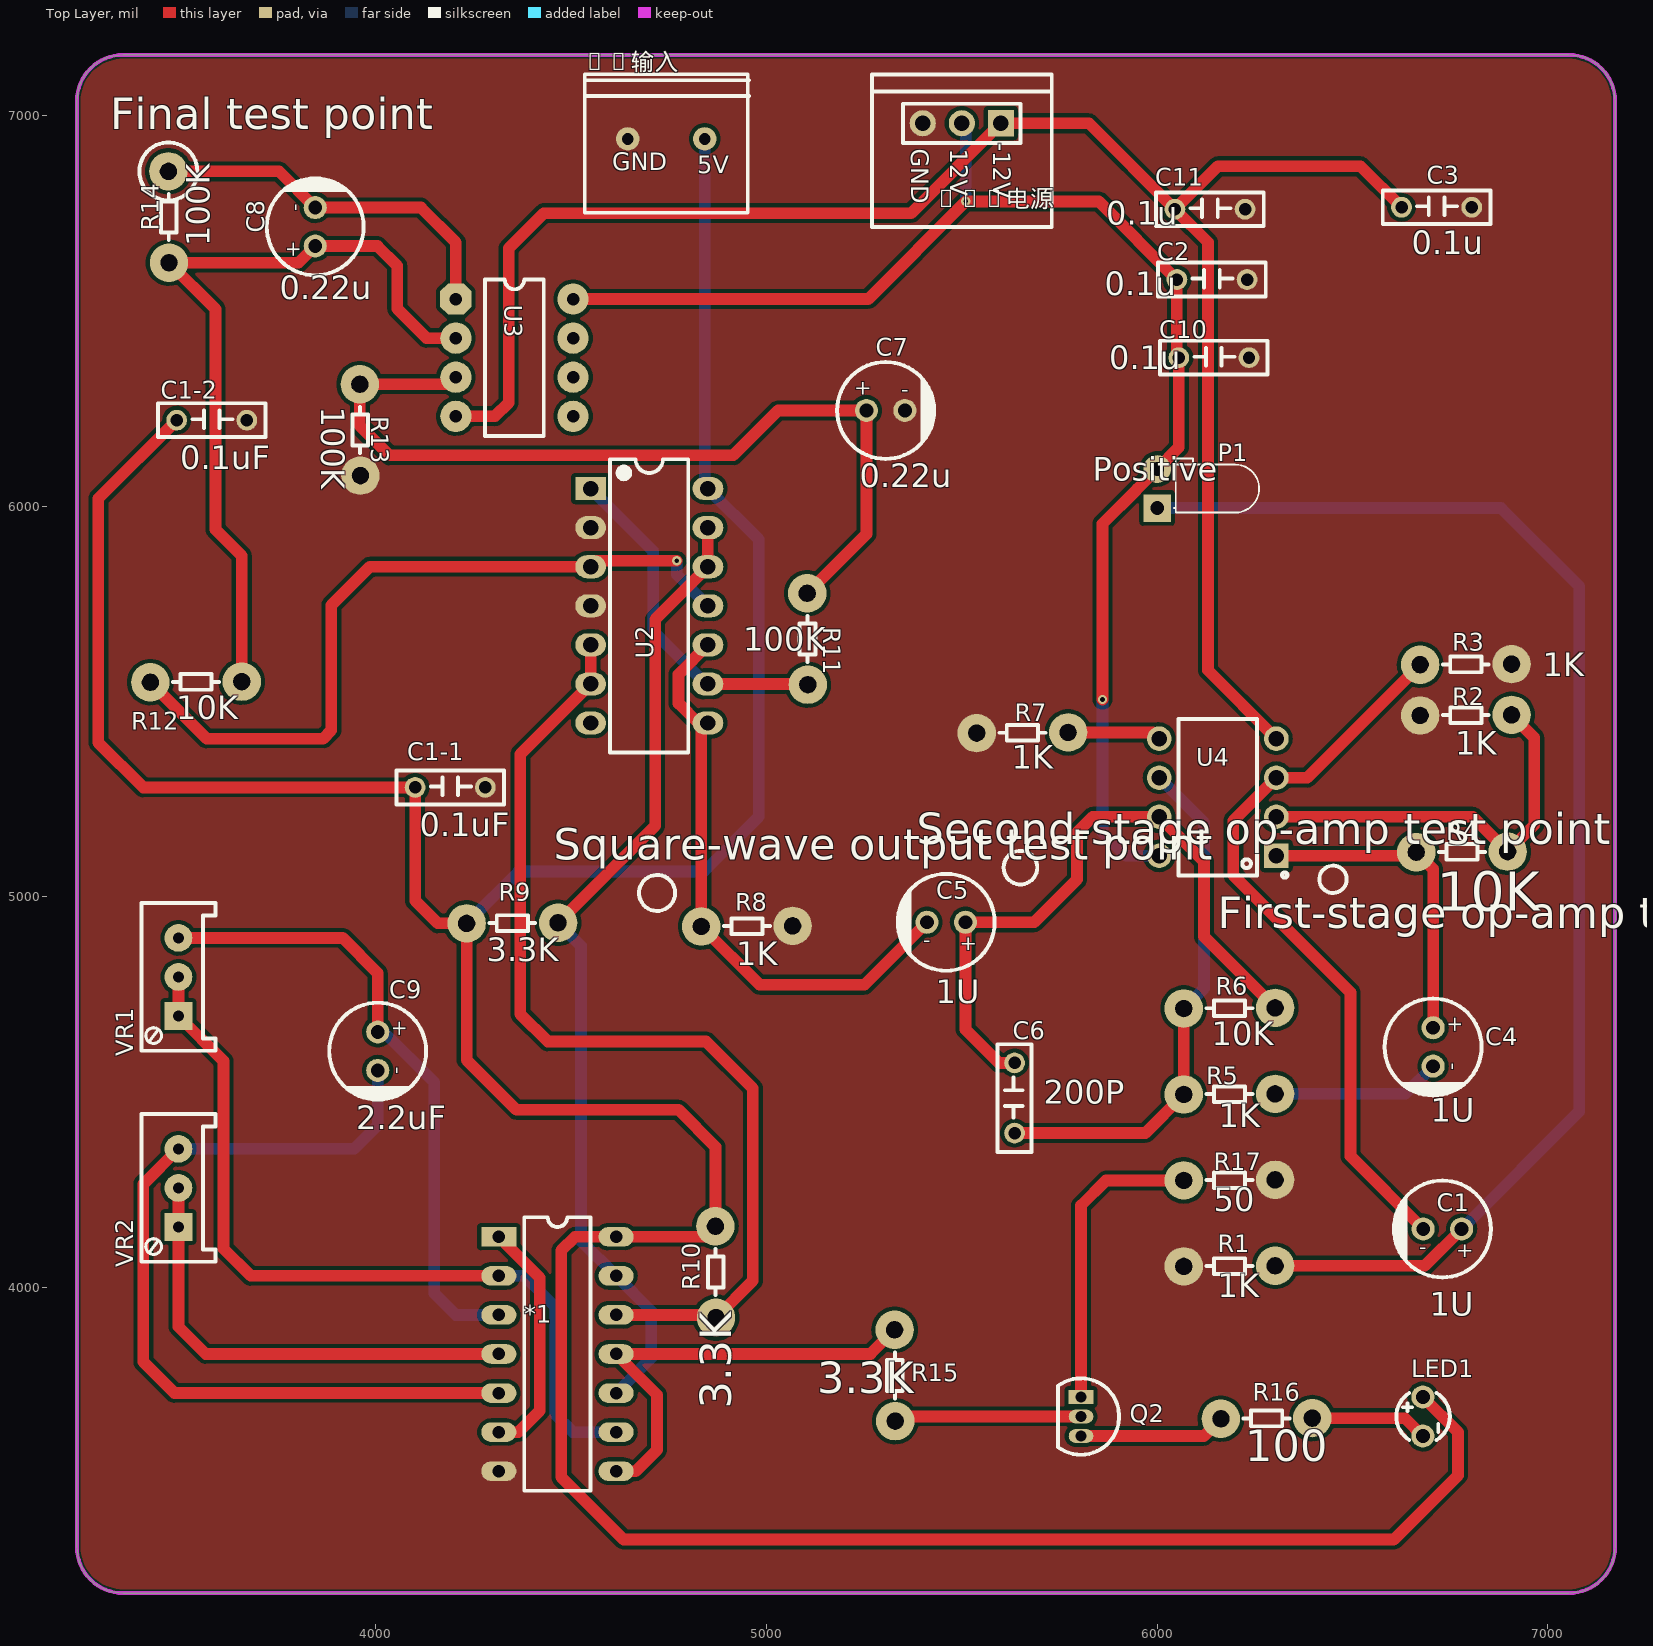
[diagram p0: Top Layer view]
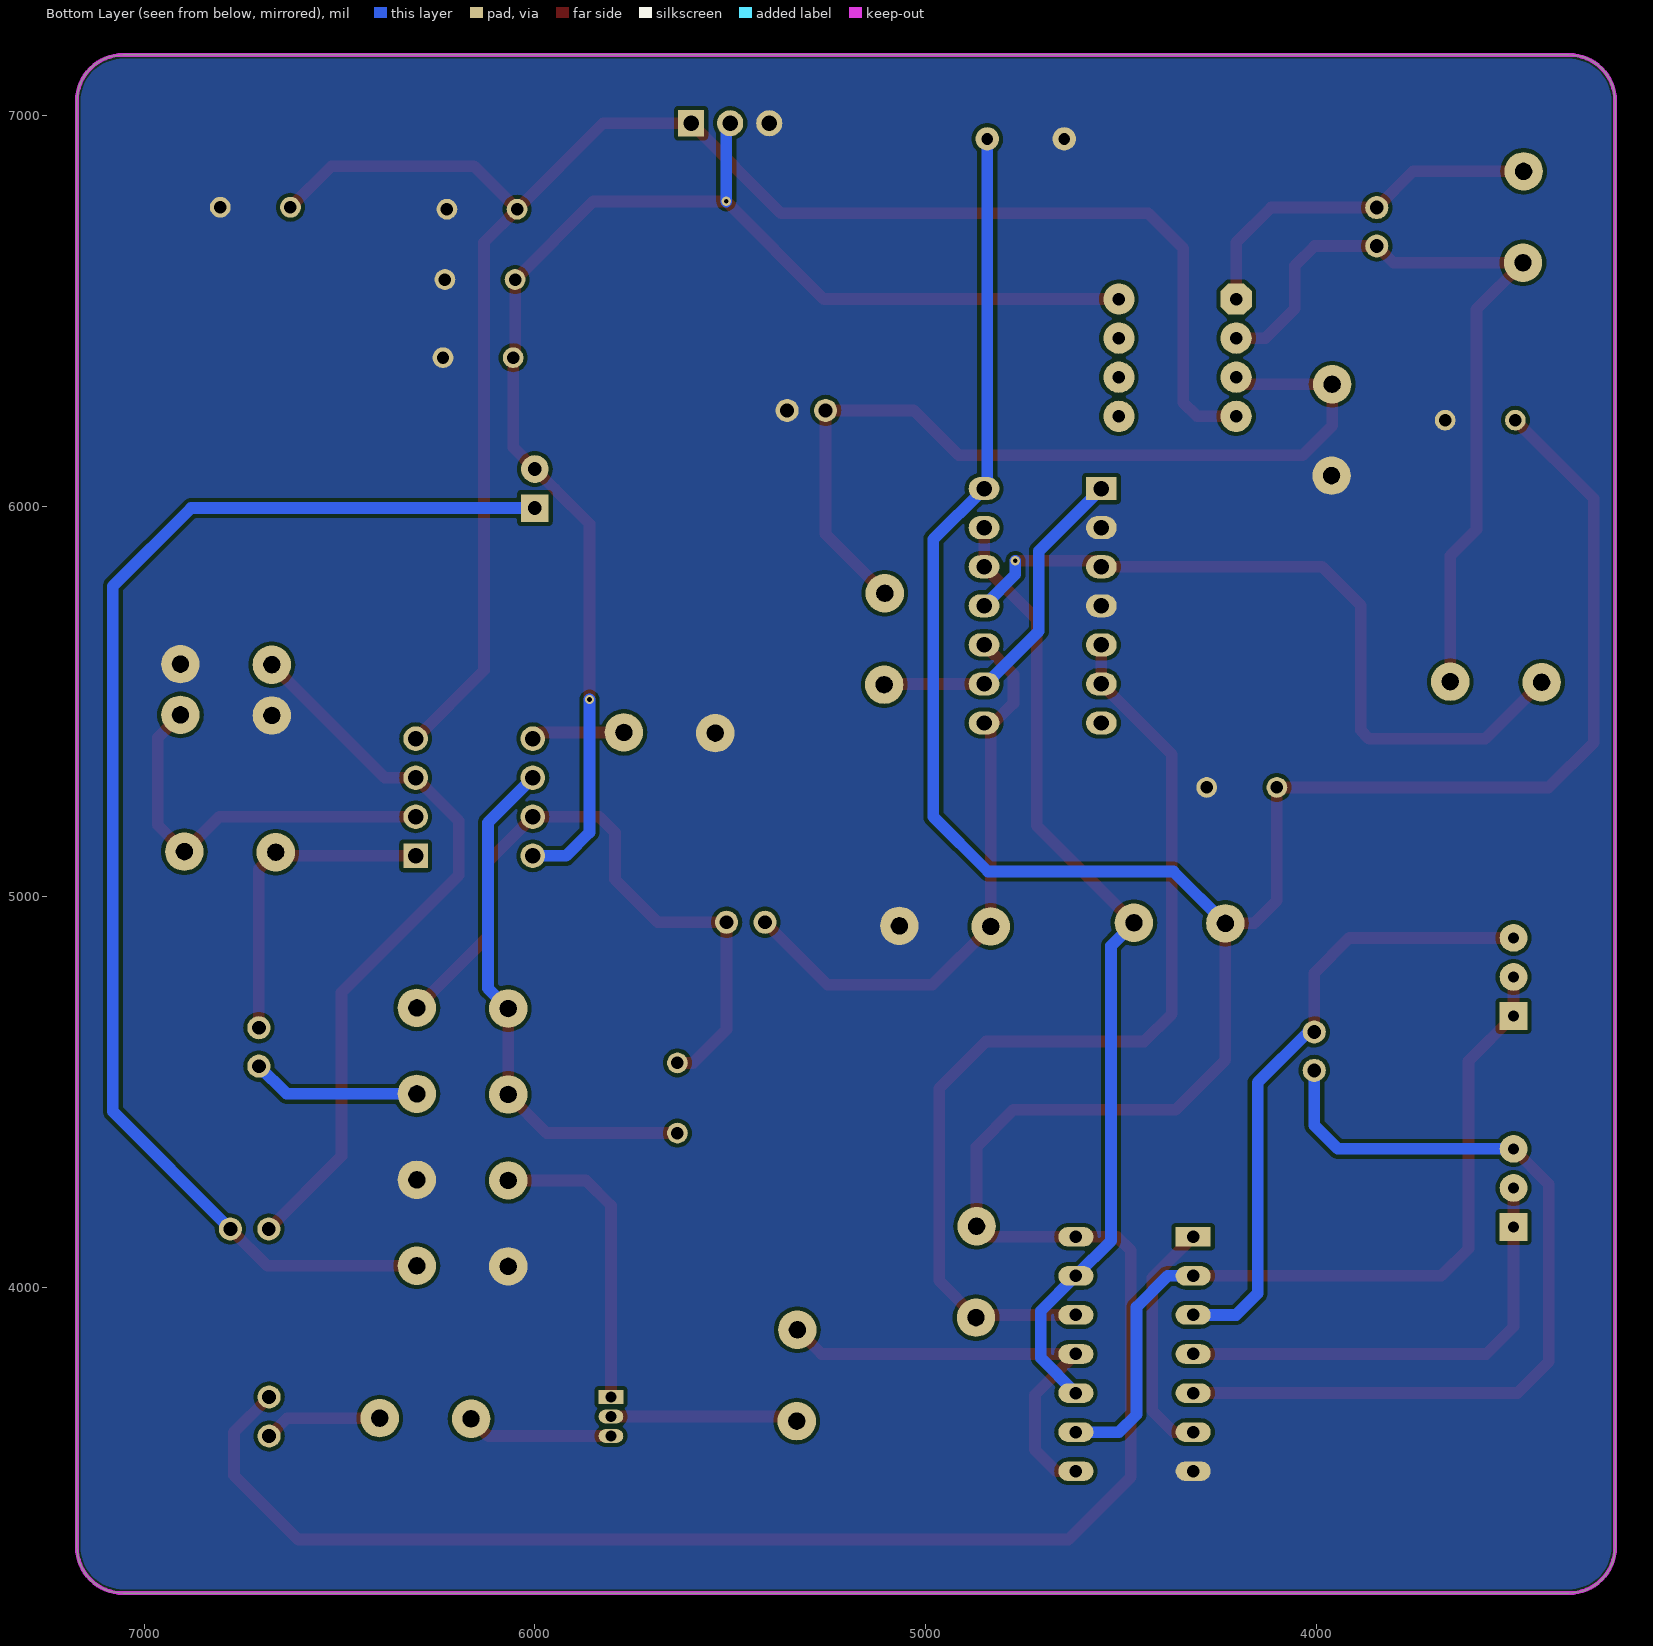
[diagram p1: Bottom Layer view, seen from below]
# Altium PCB MISC75396.pcbdoc
Units mil, origin at the board's own origin, x right, y up, seen from the top; angles counter-clockwise.
Board outline 3937.01 x 3937.01 mil, 2 copper layers (Top Layer, Bottom Layer), stack 62.206 mil thick; 41 components, 30 nets, 122 pads, 3 vias.

## Layer stack, top to bottom
Top Solder Mask Layer: solder mask 0.394, Dk 3.3
Top Layer: signal copper 1.379
Dielectric1: surface 59.449, FR4, Dk 4.5
Bottom Layer: signal copper 1.378
Bottom Solder Mask Layer: solder mask 0.394, Dk 3.3

## Board outline
3353.11,7155 ccw(c3353.11,7036.89) 3235,7036.89 3235,3336.1 ccw(c3353.11,3336.1) 3353.11,3217.99 7053.9,3217.99 ccw(c7053.9,3336.1) 7172.01,3336.1 7172.01,7036.89 ccw(c7053.9,7036.89) 7053.9,7155

## Design rules (kind name [scope] priority, off if disabled: settings)
BoardOutlineClearance copperThickness2oz_1 [All] p2 off: genericclearance=7.99 ignorepadtopadclearanceinfootprint=FALSE except(0: Arc-SplitContinuation Track-SplitContinuation SMDPad-SplitContinuation THPad-SplitContinuation Via-SplitContinuation Fill-SplitContinuation Region-SplitContinuation Poly-SplitContinuation Text-SplitContinuation Hole-SplitContinuation; 5.98: Arc-CutoutEdge Track-CutoutEdge SMDPad-CutoutEdge THPad-CutoutEdge Via-CutoutEdge Text-CutoutEdge; 6.89: Hole-OutlineEdge Hole-CutoutEdge; 10: Poly-OutlineEdge Poly-CutoutEdge; 11.81: Arc-OutlineEdge Track-OutlineEdge SMDPad-OutlineEdge THPad-OutlineEdge Via-OutlineEdge Fill-OutlineEdge Region-OutlineEdge Text-OutlineEdge Fill-CutoutEdge Region-CutoutEdge)
BoardOutlineClearance Plane_innerPlane_1 [All] p4 off: genericclearance=4.02 ignorepadtopadclearanceinfootprint=FALSE except(0: Arc-SplitContinuation Track-SplitContinuation SMDPad-SplitContinuation THPad-SplitContinuation Via-SplitContinuation Fill-SplitContinuation Region-SplitContinuation Poly-SplitContinuation Text-SplitContinuation Hole-SplitContinuation; 5.98: Arc-CutoutEdge Track-CutoutEdge SMDPad-CutoutEdge THPad-CutoutEdge Via-CutoutEdge Text-CutoutEdge; 6.89: Hole-OutlineEdge Hole-CutoutEdge; 10: Poly-OutlineEdge Poly-CutoutEdge; 11.81: Arc-OutlineEdge Track-OutlineEdge SMDPad-OutlineEdge THPad-OutlineEdge Via-OutlineEdge Fill-OutlineEdge Region-OutlineEdge Text-OutlineEdge Fill-CutoutEdge Region-CutoutEdge)
BoardOutlineClearance Copper_copperRegion_1 [All] p6 off: genericclearance=4.02 ignorepadtopadclearanceinfootprint=FALSE except(0: Arc-SplitContinuation Track-SplitContinuation SMDPad-SplitContinuation THPad-SplitContinuation Via-SplitContinuation Fill-SplitContinuation Region-SplitContinuation Poly-SplitContinuation Text-SplitContinuation Hole-SplitContinuation; 5.98: Arc-CutoutEdge Track-CutoutEdge SMDPad-CutoutEdge THPad-CutoutEdge Via-CutoutEdge Text-CutoutEdge; 6.89: Hole-OutlineEdge Hole-CutoutEdge; 10: Poly-OutlineEdge Poly-CutoutEdge; 11.81: Arc-OutlineEdge Track-OutlineEdge SMDPad-OutlineEdge THPad-OutlineEdge Via-OutlineEdge Fill-OutlineEdge Region-OutlineEdge Text-OutlineEdge Fill-CutoutEdge Region-CutoutEdge)
BoardOutlineClearance copperThickness1oz_1 [All] p8: genericclearance=4.02 ignorepadtopadclearanceinfootprint=FALSE except(0: Arc-SplitContinuation Track-SplitContinuation SMDPad-SplitContinuation THPad-SplitContinuation Via-SplitContinuation Fill-SplitContinuation Region-SplitContinuation Poly-SplitContinuation Text-SplitContinuation Hole-SplitContinuation; 5.98: Arc-CutoutEdge Track-CutoutEdge SMDPad-CutoutEdge THPad-CutoutEdge Via-CutoutEdge Text-CutoutEdge; 6.89: Hole-OutlineEdge Hole-CutoutEdge; 10: Poly-OutlineEdge Poly-CutoutEdge; 11.81: Arc-OutlineEdge Track-OutlineEdge SMDPad-OutlineEdge THPad-OutlineEdge Via-OutlineEdge Fill-OutlineEdge Region-OutlineEdge Text-OutlineEdge Fill-CutoutEdge Region-CutoutEdge)
Clearance copperThickness2oz [All] p1 off: gap=7.99 ignorepadtopadclearanceinfootprint=FALSE except(5.98: SMDPad-Track SMDPad-SMDPad THPad-Track SMDPad-THPad THPad-THPad Track-Via SMDPad-Via THPad-Via Via-Via Fill-SMDPad Region-SMDPad Fill-THPad Region-THPad Fill-Via Region-Via Fill-Fill Fill-Region Region-Region Arc-Track Arc-SMDPad Arc-THPad Arc-Via Fill-Arc Region-Arc Arc-Arc Text-Track SMDPad-Text Text-THPad Text-Via Fill-Text Region-Text Arc-Text Text-Text; 6.89: Hole-Track Hole-SMDPad Hole-THPad Hole-Via Fill-Hole Region-Hole Hole-Arc Hole-Text; 10: Poly-Track Poly-SMDPad Poly-THPad Poly-Via Poly-Fill Poly-Region Poly-Poly Poly-Arc Poly-Text Poly-Hole; 11.81: Fill-Track Region-Track)
Clearance Plane_innerPlane [All] p3 off: gap=4.02 ignorepadtopadclearanceinfootprint=FALSE except(5.98: SMDPad-Track SMDPad-SMDPad THPad-Track SMDPad-THPad THPad-THPad Track-Via SMDPad-Via THPad-Via Via-Via Fill-SMDPad Region-SMDPad Fill-THPad Region-THPad Fill-Via Region-Via Fill-Fill Fill-Region Region-Region Arc-Track Arc-SMDPad Arc-THPad Arc-Via Fill-Arc Region-Arc Arc-Arc Text-Track SMDPad-Text Text-THPad Text-Via Fill-Text Region-Text Arc-Text Text-Text; 6.89: Hole-Track Hole-SMDPad Hole-THPad Hole-Via Fill-Hole Region-Hole Hole-Arc Hole-Text; 10: Poly-Track Poly-SMDPad Poly-THPad Poly-Via Poly-Fill Poly-Region Poly-Poly Poly-Arc Poly-Text Poly-Hole; 11.81: Fill-Track Region-Track)
Clearance Copper_copperRegion [All] p5 off: gap=4.02 ignorepadtopadclearanceinfootprint=FALSE except(5.98: SMDPad-Track SMDPad-SMDPad THPad-Track SMDPad-THPad THPad-THPad Track-Via SMDPad-Via THPad-Via Via-Via Fill-SMDPad Region-SMDPad Fill-THPad Region-THPad Fill-Via Region-Via Fill-Fill Fill-Region Region-Region Arc-Track Arc-SMDPad Arc-THPad Arc-Via Fill-Arc Region-Arc Arc-Arc Text-Track SMDPad-Text Text-THPad Text-Via Fill-Text Region-Text Arc-Text Text-Text; 6.89: Hole-Track Hole-SMDPad Hole-THPad Hole-Via Fill-Hole Region-Hole Hole-Arc Hole-Text; 10: Poly-Track Poly-SMDPad Poly-THPad Poly-Via Poly-Fill Poly-Region Poly-Poly Poly-Arc Poly-Text Poly-Hole; 11.81: Fill-Track Region-Track)
Clearance copperThickness1oz [All] p7: gap=4.02 ignorepadtopadclearanceinfootprint=FALSE except(5.98: SMDPad-Track SMDPad-SMDPad THPad-Track SMDPad-THPad THPad-THPad Track-Via SMDPad-Via THPad-Via Via-Via Fill-SMDPad Region-SMDPad Fill-THPad Region-THPad Fill-Via Region-Via Fill-Fill Fill-Region Region-Region Arc-Track Arc-SMDPad Arc-THPad Arc-Via Fill-Arc Region-Arc Arc-Arc Text-Track SMDPad-Text Text-THPad Text-Via Fill-Text Region-Text Arc-Text Text-Text; 6.89: Hole-Track Hole-SMDPad Hole-THPad Hole-Via Fill-Hole Region-Hole Hole-Arc Hole-Text; 10: Poly-Track Poly-SMDPad Poly-THPad Poly-Via Poly-Fill Poly-Region Poly-Poly Poly-Arc Poly-Text Poly-Hole; 11.81: Fill-Track Region-Track)
DiffPairsRouting differentialPair [All] p1: maxlimit=6 minlimit=6 mostfreqgap=6 toplayer_minwidth=5 toplayer_prefwidth=10 toplayer_maxwidth=100 toplayer_mingap=6 toplayer_prefgap=6 toplayer_maxgap=6 bottomlayer_minwidth=5 bottomlayer_prefwidth=10 bottomlayer_maxwidth=100 bottomlayer_mingap=6 bottomlayer_prefgap=6 bottomlayer_maxgap=6 maxuncoupledlength=10
HoleToHoleClearance otherClearance [All] p1: gap=11.81 allowstackedmicrovias=TRUE
Length netLength [All] p1: minlimit=0 maxlimit=0
PasteMaskExpansion pasteMaskExpansion [All] p1: expansion=0
PlaneConnect innerPlane [All] p1: planeconnectstyle=Relief reliefexpansion=20 reliefentries=4 reliefconductorwidth=10 reliefairgap=10
PolygonConnect copperRegion [All] p1: connectstyle=Direct reliefconductorwidth=10 reliefentries=4 polygonreliefangle="90 Angle" airgapwidth=10 via.connectstyle=Relief via.reliefconductorwidth=10 via.reliefentries=4 via.polygonreliefangle="90 Angle" via.airgapwidth=10
RoutingVias viaSize [All] p1: holewidth=12.01 width=24.02 viastyle="Through Hole" minholewidth=11.81 minwidth=19.68 maxholewidth=248.03 maxwidth=393.7
SolderMaskExpansion solderMaskExpansion [IsVia] p1: expansion=-1000 istentingtop=TRUE
SolderMaskExpansion solderMaskExpansion [All] p2: expansion=2.01 istentingtop=FALSE
Width copperThickness2oz_2 [All] p1 off: maxlimit=100 minlimit=8 preferedwidth=10
Width copperThickness1oz_2 [All] p2: maxlimit=100 minlimit=5 preferedwidth=10

## Components (designator, comment, footprint, x,y, rotation, side; value= is the part's Value field where it differs from the comment)
5V输入 "5V output" 2INT 4645,6940 r0 top
12V电源 "3PIN" 3PIN 5500,6980 r0 top
*1 "74HC04" DIP14 4315.01,4129.99 r0 top
C1 "220uF" CAP-TH_BD6.3-P2.50-D0.5-FD 6730,4150 r180 top
C1-1 "" 电容直插 4190.33,5280.14 r180 top
C1-2 "" 电容直插 3580,6220 r180 top
C2 "" 电容直插 6140,6580 r180 top
C3 "" 电容直插 6715,6765 r180 top
C4 "220uF" CAP-TH_BD6.3-P2.50-D0.5-FD 6706.2,4615.85 r270 top
C5 "220uF" CAP-TH_BD6.3-P2.50-D0.5-FD 5460,4935 r180 top
C6 "" 电容直插 5635,4485 r270 top
C7 "220uF" CAP-TH_BD6.3-P2.50-D0.5-FD 5305,6245 r0 top
C8 "220uF" CAP-TH_BD6.3-P2.50-D0.5-FD 3845,6715 r90 top
C9 "220uF" CAP-TH_BD6.3-P2.50-D0.5-FD 4005,4605 r270 top
C10 "" 电容直插 6145,6380 r180 top
C11 "" 电容直插 6135,6760 r180 top
LED1 "3A4GUD" LED-TH_BD3.5-P2.54-RD-GREEN 6680,3670 r90 top
P1 "" LED_D3.0mm_Horizontal_O1.27mm_Z2.0mm 6000,6045 r90 top
Q2 "S9018" TO-92-3_L4.9-W3.7-P1.27-L 5805,3670 r270 top
R1 "" D45-V(直插) 6185,4055 r180 top
R2 "" D45-V(直插) 6790,5595 r0 top
R3 "" D45-V(直插) 6790,5465 r180 top
R4 "" D45-V(直插) 6780,5115 r0 top
R5 "" D45-V(直插) 6185,4495 r0 top
R6 "" D45-V(直插) 6185,4715 r0 top
R7 "" D45-V(直插) 5655,5420 r0 top
R8 "" D45-V(直插) 4950,4925 r0 top
R9 "" D45-V(直插) 4349.56,4932.93 r180 top
R10 "" D45-V(直插) 4870.01,4039.99 r90 top
R11 "" D45-V(直插) 5105,5660 r90 top
R12 "" D45-V(直插) 3540,5550 r0 top
R13 "" D45-V(直插) 3960,6195 r270 top
R14 "" D45-V(直插) 3470,6740 r90 top
R15 "" D45-V(直插) 5328.75,3775 r270 top
R16 "" D45-V(直插) 6280,3665 r0 top
R17 "" D45-V(直插) 6185,4275 r180 top
U2 "CD4066DN" PDIP-14_L19.3-W6.5-P2.54-LS7.6-BL 4700,5745 r270 top
U3 "LF353" DIP-8 4205,6530 r0 top
U4 "" DIP-8_L9.9-W6.4-P2.54-LS7.6-BL 6155,5255 r90 top
VR1 "101" 3296W 3495,4795 r90 top
VR2 "101" 3296W 3495,4255 r90 top

## Footprints (in the part's own frame and the unit in brackets; to place one, negate y for a bottom-side part, rotate by r counter-clockwise, add the part's x,y. Pads: shape width x height; smd on the part's side, far side on the other; paste and mask are expansions set on the pad)
2INT [mil]
  round 60 hole 30: 1(196.85,0) 2(0,0)
  silkscreen extent -110,-189 310,165
3PIN [mm]
  rect 1.7x1.7 hole 1: 1(2.54,0)
  round 1.7 hole 1: 2(0,0) 3(-2.54,0)
  silkscreen extent -3.84,-1.27 3.81,1.27
3296W [mm]
  rect 1.8x1.8 hole 0.7: 1(-2.54,0)
  round 1.8 hole 0.7: 2(0,0) 3(2.54,0)
  silkscreen extent -4.8,-2.4 4.8,2.4
CAP-TH_BD6.3-P2.50-D0.5-FD [mm]
  round 1.5 hole 0.9 paste+0 mask+0.05: 1(-1.25,0) 2(1.25,0)
  silkscreen extent -3.15,-3.15 3.21,3.15
D45-V(直插) [mm]
  round 2.5 hole 1.1 slot 1.105 at 90 deg: 1(-2.97,-0.02) 2(2.97,0.02)
  silkscreen extent -1.49,-0.51 1.49,0.51
DIP14 [mil]
  rect 90x50 hole 32: 1(0,0)
  oval 90x50 hole 32: 2(0,-100) 3(0,-200) 4(0,-300) 5(0,-400) 6(0,-500) 7(0,-600) 8(300,-600) 9(300,-500) 10(300,-400) 11(300,-300) 12(300,-200) 13(300,-100) 14(300,0)
  silkscreen extent 65,-650 235,50
DIP-8 [mil]
  oct 80x80 hole 32: 1(0,0)
  round 80 / inner round 50 / far side round 80 hole 32: 2(0,-100) 3(0,-200) 4(0,-300) 5(300,-300) 6(300,-200) 7(300,-100) 8(300,0)
  silkscreen extent 75,-350 225,50
DIP-8_L9.9-W6.4-P2.54-LS7.6-BL [mil]
  rect 63x63 hole 39.37: 1(-150,-150)
  round 63 hole 39.37: 2(-50,-150) 3(50,-150) 4(150,-150) 5(150,150) 6(50,150) 7(-50,150) 8(-150,150)
  silkscreen extent -206,-178 200,100
LED-TH_BD3.5-P2.54-RD-GREEN [mm]
  round 1.5 hole 0.9: 1(-1.27,0) 2(1.27,0)
  silkscreen extent -1.52,-1.75 1.52,1.73
LED_D3.0mm_Horizontal_O1.27mm_Z2.0mm [mm]
  rect 1.8x1.8 hole 0.9 paste+0 mask+0: 1(-1.27,0)
  round 1.8 hole 0.9 paste+0 mask+0: 2(1.27,0)
  silkscreen extent -1.56,-6.63 1.96,-1.08
PDIP-14_L19.3-W6.5-P2.54-LS7.6-BL [mm]
  rect 1.5x2 hole 1: 1(-7.62,-3.81)
  oval 1.5x2 hole 1: 2(-5.08,-3.81) 3(-2.54,-3.81) 4(0,-3.81) 5(2.54,-3.81) 6(5.08,-3.81) 7(7.62,-3.81) 8(7.62,3.81) 9(5.08,3.81) 10(2.54,3.81) 11(0,3.81) 12(-2.54,3.81) 13(-5.08,3.81) 14(-7.62,3.81)
  silkscreen extent -9.53,-2.55 9.53,2.53
TO-92-3_L4.9-W3.7-P1.27-L [mm]
  rect 0.9x1.6 hole 0.7: 1(-1.27,0)
  oval 0.9x1.6 hole 0.7: 2(0,0) 3(1.27,0)
  silkscreen extent -2.48,-1.5 2.48,2.48
电容直插 [mm]
  round 1.35 hole 0.81: 1(-2.286,0) 2(2.276,0)
  silkscreen extent -3.5,-1.1 3.5,1.1

## Via types
v1: diameter 24.02, hole 12, Top Layer to Bottom Layer, 3 vias

## Nets (pads, with @x,y where several pads share a name; then routed paths per layer and width w, separated by ;. In a path a pad name is that pad's centre, name@x,y a point inside that pad or via, vN(x,y) a via of type N, cw(c..) or ccw(c..) an arc to the next point about the centre after c; other vN are vias at no path point)
1: C4.1 R4.1 U4.1 | length 828.9
  Top Layer w30: U4.1 6653.86,5105.01 R4.1 6706.2,5071.09 C4.1
2: R3.1 R4.2 U4.2 | length 1031.1
  Top Layer w30: U4.2 6807.71,5205.01 R4.2 6965,5183.85 6965,5407.72 R3.1
3: C1.2 R2.1 U4.3 | length 1889.7
  Top Layer w30: R2.1 6383.86,5305.01 U4.3 6195,5195 6195,5055 6495,4755 6495,4335.79 C1.2
5: R7.2 U4.5 | length 239.6
  Top Layer w30: R7.2 5989.22,5420.78 U4.5
6: C6.2 R5.1 R6.1 U4.6 | length 1353.9
  Top Layer w30: C6.2 5969.24,4395.38 R5.1 R6.1
  Bottom Layer w30: U4.6 6120,5190.01 6120,4766.15 R6.1
7: C5.1 C6.1 R6.2 U4.7 | length 1725.7
  Top Layer w30: C6.1 5595,4575 5509.21,4660.79 C5.1 5685,4935 5795,5045 5795,5165 5835.01,5205.01 U4.7 6120,5090.01 6120,4897.72 R6.2
12V: 12V电源.2 C2.2 C10.2 P1.2 U3.8 U4.8 | length 3603.8
  Top Layer w30: U3.8 5260,6530 v1(5510,6780) 5850.38,6780 C2.2 6050.38,6385 C10.2 6055.38,6150.38 P1.2 5952.82,6047.82 ccw(c5964.57,6030.43) 5947.18,6042.18 5860,5955 v1(5860,5505)
  Bottom Layer w30: 12V电源.2 5510,6970 v1(5510,6780) ; v1(5860,5505) 5860,5165 5919.99,5105.01 U4.8
$1N1572: C1.1 P1.1 R1.1 | length 3448.7
  Top Layer w30: R1.1 6684.99,4055.78 C1.1
  Bottom Layer w30: P1.1 6880,5995 7080,5795 7080,4450.79 C1.1
$1N2846: C4.2 R5.2 | length 433.6
  Bottom Layer w30: R5.2 6635.34,4495.78 C4.2
$1N2910: C5.2 R8.1 U2.8 U2.10 | length 1510.4
  Top Layer w30: U2.10 4775,5570 4775,5495 4825,5445 U2.8 4833.07,5428.07 R8.1 4982.28,4775 5250.79,4775 C5.2
$1N2968: R11.1 U2.1 U2.9 | length 883.8
  Top Layer w30: U2.9 5103.85,5545 R11.1
  Bottom Layer w30: U2.1 4710,5885 4710,5680 4845,5545 U2.9
$1N3169: R12.1 U2.3 U2.11 | length 1930.7
  Top Layer w30: R12.1 3567.28,5405 3865,5405 3886.21,5426.21 3886.21,5746.21 3985,5845 U2.3 4565,5860 v1(4770,5860)
  Bottom Layer w30: v1(4770,5860) 4770,5825 U2.11
$1N3229: C8.1 R12.2 R14.1 U3.2 | length 2063.4
  Top Layer w30: R12.2 3656.93,5873.07 3590,5940 3590,6503.85 R14.1 3802.28,6623.07 C8.1 4004.21,6665.79 4055,6615 4055,6505 4130,6430 U3.2
$1N3233: C7.1 R11.2 R13.1 U3.3 | length 2265.9
  Top Layer w30: U3.3 4186.93,6311.93 R13.1 3959.22,6205.78 4035,6130 4915,6130 5030,6245 C7.1 5255.79,5928.51 R11.2
$1N3822: *1.12 R10.1 U2.5 U2.6 | length 2577.9
  Top Layer w30: U2.5 U2.6 4370,5365 4370,4700 4440,4630 4845,4630 4965,4510 4965,4017.27 R10.1 4863.86,3929.99 *1.12
$1N4613: *1.10 *1.13 R9.1 U2.12 U2.13 | length 2509.9
  Top Layer w30: R9.1 4715,5182.22 4715,5710 U2.12 U2.13
  Bottom Layer w30: R9.1 4525,4875.2 4525,4120 *1.13 4705,3940 4705,3819.99 *1.10
$1N4655: *1.8 *1.11 R15.1 | length 1154.9
  Top Layer w30: *1.8 4664.99,3529.99 4720,3585 4720,3725 *1.11 5266.03,3829.99 R15.1
$1N4661: *1.1 *1.6 | length 616.3
  Top Layer w30: *1.6 4364.99,3629.99 4420,3685 4420,4025 *1.1
$1N4668: *1.2 *1.9 VR1.1 VR1.2 | length 2103.4
  Top Layer w30: VR1.2 VR1.1 3610,4580 3610,4100 3680.01,4029.99 *1.2
  Bottom Layer w30: *1.2 4380.01,4029.99 4460,3950 4460,3675 4505.01,3629.99 *1.9
$1N4723: *1.3 C9.1 VR1.3 | length 1624.4
  Top Layer w30: VR1.3 3915,4895 4005,4805 C9.1
  Bottom Layer w30: C9.1 4020.79,4654.21 4150,4525 4150,3985 4205.01,3929.99 *1.3
$1N4812: *1.5 C9.2 VR2.3 | length 2201.1
  Top Layer w30: VR2.3 3405,4265 3405,3810 3485.01,3729.99 *1.5
  Bottom Layer w30: VR2.3 3945,4355 4005,4415 C9.2
$1N4856: *1.4 VR2.1 VR2.2 | length 1204
  Top Layer w30: VR2.2 VR2.1 3495,3900 3565.01,3829.99 *1.4
$1N5161: LED1.1 R16.2 | length 302
  Top Layer w30: R16.2 6634.22,3665.78 LED1.1
$1N5332: Q2.2 R15.2 | length 480.4
  Top Layer w30: R15.2 5341.47,3670 Q2.2
$1N5334: Q2.3 R16.1 | length 376.4
  Top Layer w30: Q2.3 6118.85,3620 R16.1
$1N5336: Q2.1 R17.2 | length 779.7
  Top Layer w30: Q2.1 5805,4210 5869.22,4274.22 R17.2
+5V: 5V输入.1 *1.14 C1-1.2 C1-2.2 LED1.2 R9.2 R10.2 U2.14 | length 9813.7
  Top Layer w30: C1-2.2 3290,6019.62 3290,5395 3404.86,5280.14 C1-1.2 4100.72,4990.08 4158.65,4932.14 R9.2 4232.63,4582.37 4360,4455 4775,4455 4869.22,4360.78 R10.2 4842.29,4129.99 *1.14 4509.99,4129.99 4475,4095 4475,3515 4635,3355 6605,3355 6770,3520 6770,3630 LED1.2
  Bottom Layer w30: R9.2 4365.49,5065 4840,5065 4980,5205 4980,5915 U2.14 4841.85,6053.15 5V输入.1
-12V: 12V电源.1 C3.2 C11.2 U3.4 U4.4 | length 4605.1
  Top Layer w30: U3.4 4305,6230 4340,6265 4340,6660 4430,6750 5370,6750 12V电源.1 5825.38,6980 C11.2 ; U4.4 6130,5580.01 6130,6675.38 C11.2 ; C3.2 6520.38,6870 6155.38,6870 C11.2
GND: 5V输入.2 12V电源.3 *1.7 C1-1.1 C1-2.1 C2.1 C3.1 C7.2 C10.1 C11.1 R1.2 R2.2 R3.2 R7.1 R8.2 R13.2 R17.1 U2.2 U2.4
OUT: C8.2 R14.2 U3.1 | length 956.1
  Top Layer w30: R14.2 3752.28,6856.93 C8.2 4115.79,6764.21 4205,6675 U3.1
pads on no net: U2.7 U3.5 U3.6 U3.7

## Polygon pours and split planes (outlines as drawn)
GND on Top Layer (solid, remove dead copper, pour order 0): 3015,7405 3015,3000 7360,3000 7360,7405
GND on Bottom Layer (solid, remove dead copper, pour order 2): 3000,7520 3000,3010 7725,3010 7725,7520

## Keep-outs
Board Outline Layer:
  the board outline again, w10

## Silkscreen, mask and mechanical layers (free items; w line width, h text height)
Top Silkscreen Layer:
  circle w10: c6450,5045 r35
  circle w10: c5650,5075 r43.01
  circle w10: c4720,5010 r46.1
  circle w10: c3469.22,6856.93 r74.1
  lines w10: 5270,7061.6 5730,7061.6 ; 5270,6715 5270,7105 5730,7105 5730,6715 5270,6715
  text "Final test point" at 3320,6965 h80
  text "-12V" at 5580,6930 h45 r270
  text "GND" at 5370,6915 h45 r270
  text "12V" at 5470,6915 h45 r270
  text "GND" at 4605,6860 h45
  text "5V" at 4822.5,6852.5 h45
  text "0.1u" at 5870,6720 h60
  text "100K" at 3575,6665 h60 r90
  text "0.1u" at 6651.25,6645 h60
  text "0.1u" at 5866.25,6540 h60
  text "0.22u" at 3754.6,6530 h60
  text "0.1u" at 5876.87,6350 h60
  text "100K" at 3860,6255 h60 r270
  text "0.1uF" at 3499.6,6094.79 h60
  text "Positive" at 5835,6065 h60
  text "0.22u" at 5239.05,6048.74 h60
  text "100K" at 4940.56,5630 h60
  text "1K" at 6987.01,5565 h60
  text "10K" at 3489.05,5455 h60
  text "1K" at 6762.65,5364.1 h60
  text "1K" at 5627.65,5328.52 h60
  text "0.1uF" at 4112.8,5155 h60
  text "Second-stage op-amp test point" at 5385,5135 h80
  text "Square-wave output test point" at 4455,5095 h80
  text "10K" at 6715,4965 h100
  text "First-stage op-amp test point" at 6155,4920 h80
  text "3.3K" at 4283.61,4835.17 h60
  text "1K" at 4922.65,4824.78 h60
  text "1U" at 5432.65,4728.22 h60
  text "10K" at 6140,4620 h60
  text "200P" at 5710,4470 h60
  text "1U" at 6700,4425 h60
  text "1K" at 6157.65,4410 h60
  text "2.2uF" at 3950,4405 h60
  text "50" at 6145,4195 h60
  text "1K" at 6155,3975 h60
  text "1U" at 6697.54,3928.07 h60
  text "3.3K" at 5130,3730 h80
  text "3.3K" at 4910.01,3689.99 h80 r90
  text "100" at 6225,3555 h80